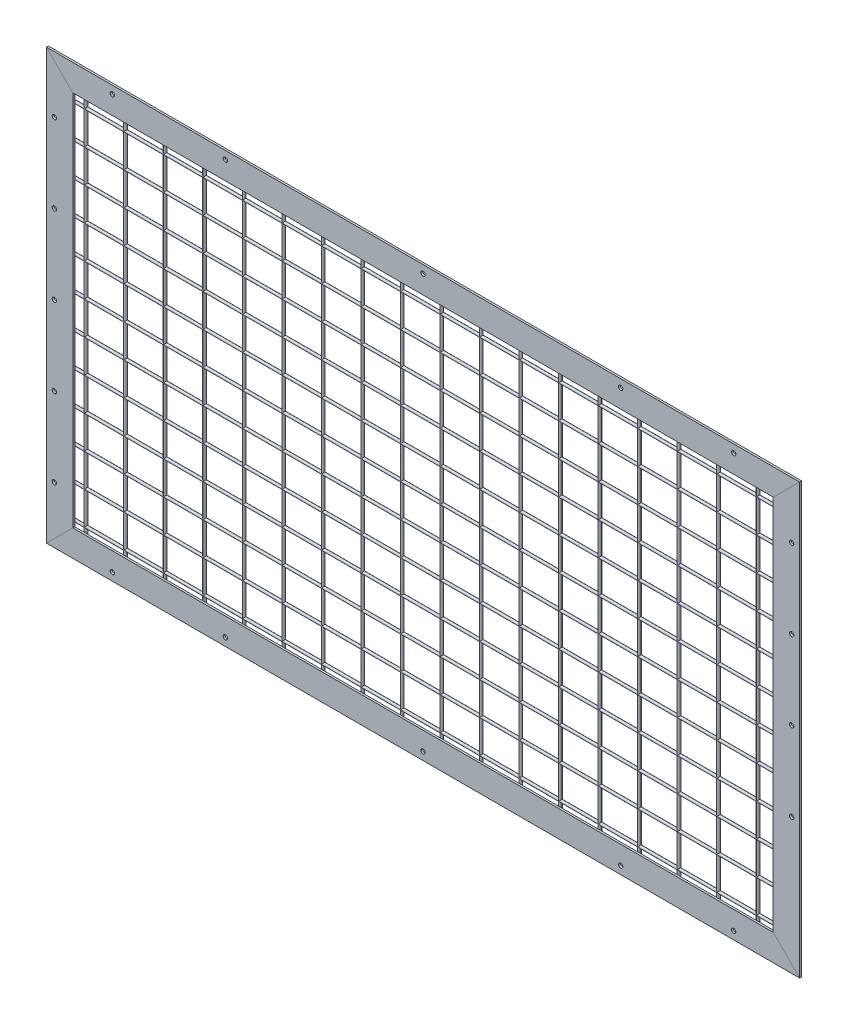
SolidWorks part; units mm, degrees
material "Q235-A GB/T700-2006"
material "Q235-A GB/T700-2006"
material "Q235-A GB/T700-2006"
material "Q235-A GB/T700-2006"
material "Q235-A GB/T700-2006"
material "Q235-A GB/T700-2006"
ref_plane "前视" through (0, 0, 0) normal (0, 0, 1) x (1, 0, 0)
ref_plane "上视" through (0, 0, 0) normal (0, 1, 0) x (1, 0, 0)
ref_plane "右视" through (0, 0, 0) normal (1, 0, 0) x (0, 0, -1)
sketch "草图4" plane through (0, 0, 0) normal (0, 0, 1) x (1, 0, 0)
  line L1 (0, 0) -> (40, 40)
  line L2 (0, 0) -> (0, 652)
  line L3 (0, 652) -> (40, 612)
  line L4 (40, 40) -> (40, 612)
  line L5 (1103, 40) -> (1143, 0)
  line L6 (1103, 40) -> (1103, 612)
  line L7 (1103, 612) -> (1143, 652)
  line L8 (1143, 0) -> (1143, 652)
  dimension "D1" = 652
  dimension "D2" = 45
  dimension "D3" = 1143
  dimension "D4" = 40
  dimension "D5" = 45
  dimension "D6" = 45
  dimension "D7" = 45
extrude "凸台-拉伸2" add sketch "草图4" along normal blind 3
sketch "草图6" plane through (0, 0, 3) normal (0, 0, 1) x (1, 0, 0)
  line L0 (1103, 612) -> (1103, 40) construction
  line L1 (0, 0) -> (1143, 0)
  line L2 (0, 0) -> (40, 40)
  line L3 (40, 40) -> (1103, 40)
  line L4 (1143, 0) -> (1103, 40)
  line L5 (40, 612) -> (0, 652) construction
  line L6 (0, 652) -> (1143, 652)
  line L7 (0, 652) -> (40, 612)
  line L8 (40, 612) -> (1103, 612)
  line L9 (1143, 652) -> (1103, 612)
  line L10 (1143, 0) -> (1143, 652) construction
  line L11 (1143, 652) -> (1103, 612) construction
  line L12 (0, 0) -> (40, 40) construction
extrude "凸台-拉伸3" add sketch "草图6" against normal up to surface (3 mm away) separate body up to face at (20, 326, 0)
ref_plane "基准面1" through (0, 25, 0) normal (0, -1, 0) x (-1, 0, 0)
ref_plane "基准面2" through (25, 0, 0) normal (-1, 0, 0) x (0, 0, 1)
sketch "草图7" plane through (0, 25, 0) normal (0, -1, 0) x (-1, 0, 0)
  line L0 (0, 0) -> (-1143, 0) construction
  line L1 (0, -3) -> (0, 0) construction
  circle A0 centre (-55, 2) radius 2
  circle A1 centre (-115, 2) radius 2
  circle A2 centre (-175, 2) radius 2
  circle A3 centre (-235, 2) radius 2
  circle A4 centre (-295, 2) radius 2
  circle A5 centre (-355, 2) radius 2
  circle A6 centre (-415, 2) radius 2
  circle A7 centre (-475, 2) radius 2
  circle A8 centre (-535, 2) radius 2
  circle A9 centre (-595, 2) radius 2
  circle A10 centre (-655, 2) radius 2
  circle A11 centre (-715, 2) radius 2
  circle A12 centre (-775, 2) radius 2
  circle A13 centre (-835, 2) radius 2
  circle A14 centre (-895, 2) radius 2
  circle A15 centre (-955, 2) radius 2
  circle A16 centre (-1015, 2) radius 2
  circle A17 centre (-1075, 2) radius 2
  circle A20 centre (-1195, 2) radius 2 [skipped]
  circle A21 centre (-1135, 2) radius 2 [skipped]
  dimension "D1" = 4
  dimension "D2" = 55
  dimension "D3" = 20
extrude "凸台-拉伸4" add sketch "草图7" against normal offset from surface (602 mm away) 25 separate body up to face at (571.5, 652, 1.5)
sketch "草图8" plane through (25, 0, 0) normal (-1, 0, 0) x (0, 0, 1)
  line L0 (0, 652) -> (0, 0) construction
  line L2 (-4, 25) -> (0, 25) construction
  circle A0 centre (-2, 47.1) radius 2
  circle A1 centre (-2, 97.1) radius 2
  circle A2 centre (-2, 147.1) radius 2
  circle A3 centre (-2, 197.1) radius 2
  circle A4 centre (-2, 247.1) radius 2
  circle A5 centre (-2, 297.1) radius 2
  circle A6 centre (-2, 347.1) radius 2
  circle A7 centre (-2, 397.1) radius 2
  circle A8 centre (-2, 447.1) radius 2
  circle A9 centre (-2, 497.1) radius 2
  circle A10 centre (-2, 547.1) radius 2
  circle A11 centre (-2, 597.1) radius 2
  circle A15 centre (-2, 647.1) radius 2 [skipped]
  circle A16 centre (-2, 697.1) radius 2 [skipped]
  circle A17 centre (-2, 747.1) radius 2 [skipped]
  dimension "D1" = 4
  dimension "D2" = 22.1
  dimension "D4" = 5
  dimension "D3" = 11
extrude "凸台-拉伸5" add sketch "草图8" against normal offset from surface (1093 mm away) 25 up to face at (1143, 326, 1.5)
hole_wizard "M6 间隙孔1" positions "草图10" profile "草图9" hole size "M6" standard "ISO" end condition up to next
sketch "草图10" plane through (0, 0, 3) normal (0, 0, 1) x (1, 0, 0)
  line L0 (0, 326) -> (-547.7626, 326) construction
  line L1 (0, 652) -> (0, 0) construction
  line L4 (571.5, 0) -> (571.5, 640) construction
  line L5 (1143, 652) -> (0, 652) construction
  line L6 (0, 0) -> (1143, 0) construction
  point P0 (100, 640)
  point P2 (571.5, 640)
  point P12 (12, 566)
  point P35 (12, 86)
  point P36 (1043, 12)
  point P37 (571.5, 12)
  point P38 (100, 12)
  point P48 (271.5, 640)
  point P50 (271.5, 12)
  point P54 (871.5, 12)
  point P61 (12, 446)
  point P63 (12, 326)
  point P65 (12, 206)
  point P72 (1131, 446)
  point P74 (1131, 326)
  point P76 (1131, 206)
  point P86 (871.5, 640)
  point P89 (1043, 640)
  point P91 (1131, 566)
  dimension "D1" = 12
  dimension "D2" = 100
  dimension "D3" = 120
  dimension "D4" = 12
  dimension "D5" = 300
  dimension "D7" = 240
sketch "草图9" plane through (100, 640, 3) normal (1, 0, 0) x (0, -1, 0)
  line L0 (0, 0) -> (0, 3.001)
  line L1 (0, 3.001) -> (3.3, 3.001)
  line L2 (3.3, 3.001) -> (3.3, 0)
  line L5 (3.3, 0) -> (0, 0)
  line L11 (0, -6.35) -> (0, 107.95) construction
  dimension "通孔孔直径" = 6.6
  dimension "通孔孔深度" = 3.001
sketch "草图11" plane through (0, 0, 3) normal (0, 0, 1) x (1, 0, 0)
  line L1 (1143, 0) -> (1060, 0)
  line L2 (1143, 0) -> (1143, 158)
  line L3 (1143, 158) -> (1060, 158)
  line L4 (1060, 0) -> (1060, 158)
  dimension "D1" = 83
  dimension "D2" = 158
extrude "切除-拉伸1" [suppressed] cut sketch "草图11" against normal blind 10
sketch "草图14" plane through (0, 0, 3) normal (0, 0, 1) x (1, 0, 0)
  line L0 (1143, 652) -> (0, 652) construction
  line L1 (1143, 0) -> (1103, 0)
  line L2 (1143, 0) -> (1143, 652)
  line L3 (1143, 652) -> (1103, 652)
  line L4 (1103, 0) -> (1103, 652)
  dimension "D1" = 40
extrude "切除-拉伸4" [suppressed] cut sketch "草图14" against normal blind 433
